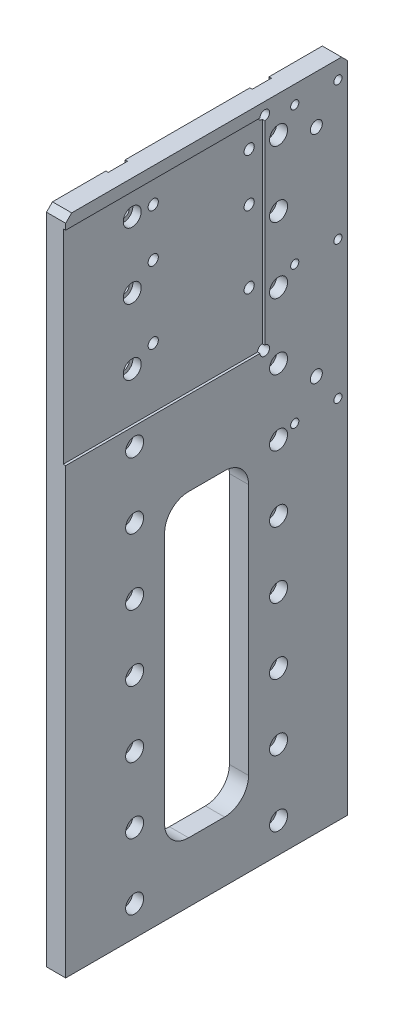
from build123d import *

# Parameters (mm, degrees)
SKETCH_1_W               = 16
SKETCH_1_H               = 550
EXTRUDE_1_DEPTH          = 235
SKETCH_4_W               = 16
SKETCH_4_H               = 550
CUT_EXTRUDE_3_DEPTH      = 2
SKETCH_5_W               = 166
SKETCH_5_H               = 170
CUT_EXTRUDE_4_DEPTH      = 2
HOLE_WIZARD_M10_1_D      = 8.5
HOLE_WIZARD_M10_1_DEPTH  = 27.5
HOLE_WIZARD_M10_1_TIP    = 2.553657631
HOLE_WIZARD_M8_1_D       = 6.8
HOLE_WIZARD_M8_1_DEPTH   = 25
HOLE_WIZARD_M8_1_TIP     = 2.042926105
SKETCH_15_W              = 70
SKETCH_15_H              = 250
CUT_EXTRUDE_5_DEPTH      = 16
FILLET_1_R               = 20
CHAMFER_1_SIZE           = 5
HOLE_WIZARD_1_AT_2_COUNT = 2
HOLE_WIZARD_1_AT_2_PITCH = 120
PATTERN_LINEAR_1_COUNT   = 10
PATTERN_LINEAR_1_PITCH   = 55
HOLE_WIZARD_M8_2_D       = 6.8
HOLE_WIZARD_M8_2_DEPTH   = 22.25
HOLE_WIZARD_M8_2_TIP     = 2.042926105
SKETCH_20_R              = 4
CUT_EXTRUDE_6_DEPTH      = 363.085625232
MM_1_D                   = 10
MM_1_DEPTH               = 10
MM_1_TIP                 = 3.004303095


with BuildPart() as part:
    # 草图1 → 凸台-拉伸1 (new body)
    with BuildSketch(Plane.XY):
        Rectangle(SKETCH_1_W, SKETCH_1_H)
    extrude(amount=EXTRUDE_1_DEPTH)

    # 草图4 → 切除-拉伸3 (cut)
    with BuildSketch(Plane.ZY.offset(8)):
        with Locations((57.5, 0)):
            Rectangle(SKETCH_4_W, SKETCH_4_H)
        with Locations((177.5, 0)):
            Rectangle(SKETCH_4_W, SKETCH_4_H)
    extrude(amount=-CUT_EXTRUDE_3_DEPTH, mode=Mode.SUBTRACT)

    # 草图5 → 切除-拉伸4 (cut)
    with BuildSketch(Plane(origin=(8, 0, 0), x_dir=(0, 0, -1), z_dir=(1, 0, 0))):
        with Locations((-152, 180)):
            Rectangle(SKETCH_5_W, SKETCH_5_H)
    extrude(amount=-CUT_EXTRUDE_4_DEPTH, mode=Mode.SUBTRACT)

    # M10 螺纹孔1
    with Locations(Plane(origin=(6, 0, 0), x_dir=(0, 0, -1), z_dir=(1, 0, 0))):
        with Locations((-160, 245), (-80, 145), (-160, 145), (-80, 245), (-80, 205), (-160, 205)):
            Hole(HOLE_WIZARD_M10_1_D / 2, depth=HOLE_WIZARD_M10_1_DEPTH)
            with Locations((0, 0, -(HOLE_WIZARD_M10_1_DEPTH + HOLE_WIZARD_M10_1_TIP / 2))):  # 118° drill point
                Cone(0, HOLE_WIZARD_M10_1_D / 2, HOLE_WIZARD_M10_1_TIP, mode=Mode.SUBTRACT)

    # M8 螺纹孔1
    with Locations(Plane(origin=(0, -275, 0), x_dir=(-1, 0, 0), z_dir=(0, -1, 0))):
        with Locations((0, -207.5), (0, -72.5), (0, -27.5), (0, -117.5), (0, -162.5)):
            Hole(HOLE_WIZARD_M8_1_D / 2, depth=HOLE_WIZARD_M8_1_DEPTH)
            with Locations((0, 0, -(HOLE_WIZARD_M8_1_DEPTH + HOLE_WIZARD_M8_1_TIP / 2))):  # 118° drill point
                Cone(0, HOLE_WIZARD_M8_1_D / 2, HOLE_WIZARD_M8_1_TIP, mode=Mode.SUBTRACT)

    # 草图15 → 切除-拉伸5 (cut)
    with BuildSketch(Plane.ZY.offset(8)):
        with Locations((117.5, -100)):
            Rectangle(SKETCH_15_W, SKETCH_15_H)
    extrude(amount=-CUT_EXTRUDE_5_DEPTH, mode=Mode.SUBTRACT)

    # 圆角1
    fillet_1_edges = [part.edges().sort_by_distance(p)[0] for p in [
        (0, 25, 152.5),
        (0, -225, 152.5),
        (0, -225, 82.5),
        (0, 25, 82.5),
    ]]
    fillet(fillet_1_edges, radius=FILLET_1_R)

    # 倒角1
    chamfer_1_edges = [part.edges().sort_by_distance(p)[0] for p in [
        (0, 275, 0),
        (0, 275, 235),
    ]]
    chamfer(chamfer_1_edges, length=CHAMFER_1_SIZE)

    # 草图17 → 打孔尺寸(%根据)内六角圆柱头螺钉的类型1 (revolve, cut)
    with BuildSketch(Plane(origin=(8, -250, 57.5), x_dir=(0, 0, -1), z_dir=(0, 1, 0))):
        Polygon((0, 0), (0, 30.203872786), (4.5, 27.5), (4.5, 9), (7.5, 9), (7.5, 0), align=None)
    hole_wizard_1 = revolve(axis=Axis((14.35, -250, 57.5), (-1, 0, 0)), mode=Mode.SUBTRACT)

    # 打孔尺寸(%根据)内六角圆柱头螺钉的类型1 at 2: 打孔尺寸(%根据)内六角圆柱头螺钉的类型1 ×2
    with Locations(*[(0, 0, i * HOLE_WIZARD_1_AT_2_PITCH) for i in range(1, HOLE_WIZARD_1_AT_2_COUNT)]):
        add(hole_wizard_1, mode=Mode.SUBTRACT)

    # 阵列(线性)1: 打孔尺寸(%根据)内六角圆柱头螺钉的类型1 ×10
    with Locations(*[(0, i * PATTERN_LINEAR_1_PITCH, 0) for i in range(1, PATTERN_LINEAR_1_COUNT)]):
        add(hole_wizard_1, mode=Mode.SUBTRACT)

    # 阵列(线性)1 copy 1 sketch → 阵列(线性)1 copy 1 (revolve, cut)
    with BuildSketch(Plane(origin=(8, -195, 177.5), x_dir=(0, 0, -1), z_dir=(0, 1, 0))):
        Polygon((0, 0), (0, 30.203872786), (4.5, 27.5), (4.5, 9), (7.5, 9), (7.5, 0), align=None)
    revolve(axis=Axis((14.35, -195, 177.5), (-1, 0, 0)), mode=Mode.SUBTRACT)

    # 阵列(线性)1 copy 2 sketch → 阵列(线性)1 copy 2 (revolve, cut)
    with BuildSketch(Plane(origin=(8, -140, 177.5), x_dir=(0, 0, -1), z_dir=(0, 1, 0))):
        Polygon((0, 0), (0, 30.203872786), (4.5, 27.5), (4.5, 9), (7.5, 9), (7.5, 0), align=None)
    revolve(axis=Axis((14.35, -140, 177.5), (-1, 0, 0)), mode=Mode.SUBTRACT)

    # 阵列(线性)1 copy 3 sketch → 阵列(线性)1 copy 3 (revolve, cut)
    with BuildSketch(Plane(origin=(8, -85, 177.5), x_dir=(0, 0, -1), z_dir=(0, 1, 0))):
        Polygon((0, 0), (0, 30.203872786), (4.5, 27.5), (4.5, 9), (7.5, 9), (7.5, 0), align=None)
    revolve(axis=Axis((14.35, -85, 177.5), (-1, 0, 0)), mode=Mode.SUBTRACT)

    # 阵列(线性)1 copy 4 sketch → 阵列(线性)1 copy 4 (revolve, cut)
    with BuildSketch(Plane(origin=(8, -30, 177.5), x_dir=(0, 0, -1), z_dir=(0, 1, 0))):
        Polygon((0, 0), (0, 30.203872786), (4.5, 27.5), (4.5, 9), (7.5, 9), (7.5, 0), align=None)
    revolve(axis=Axis((14.35, -30, 177.5), (-1, 0, 0)), mode=Mode.SUBTRACT)

    # 阵列(线性)1 copy 5 sketch → 阵列(线性)1 copy 5 (revolve, cut)
    with BuildSketch(Plane(origin=(8, 25, 177.5), x_dir=(0, 0, -1), z_dir=(0, 1, 0))):
        Polygon((0, 0), (0, 30.203872786), (4.5, 27.5), (4.5, 9), (7.5, 9), (7.5, 0), align=None)
    revolve(axis=Axis((14.35, 25, 177.5), (-1, 0, 0)), mode=Mode.SUBTRACT)

    # 阵列(线性)1 copy 6 sketch → 阵列(线性)1 copy 6 (revolve, cut)
    with BuildSketch(Plane(origin=(8, 80, 177.5), x_dir=(0, 0, -1), z_dir=(0, 1, 0))):
        Polygon((0, 0), (0, 30.203872786), (4.5, 27.5), (4.5, 9), (7.5, 9), (7.5, 0), align=None)
    revolve(axis=Axis((14.35, 80, 177.5), (-1, 0, 0)), mode=Mode.SUBTRACT)

    # 阵列(线性)1 copy 7 sketch → 阵列(线性)1 copy 7 (revolve, cut)
    with BuildSketch(Plane(origin=(8, 135, 177.5), x_dir=(0, 0, -1), z_dir=(0, 1, 0))):
        Polygon((0, 0), (0, 30.203872786), (4.5, 27.5), (4.5, 9), (7.5, 9), (7.5, 0), align=None)
    revolve(axis=Axis((14.35, 135, 177.5), (-1, 0, 0)), mode=Mode.SUBTRACT)

    # 阵列(线性)1 copy 8 sketch → 阵列(线性)1 copy 8 (revolve, cut)
    with BuildSketch(Plane(origin=(8, 190, 177.5), x_dir=(0, 0, -1), z_dir=(0, 1, 0))):
        Polygon((0, 0), (0, 30.203872786), (4.5, 27.5), (4.5, 9), (7.5, 9), (7.5, 0), align=None)
    revolve(axis=Axis((14.35, 190, 177.5), (-1, 0, 0)), mode=Mode.SUBTRACT)

    # 阵列(线性)1 copy 9 sketch → 阵列(线性)1 copy 9 (revolve, cut)
    with BuildSketch(Plane(origin=(8, 245, 177.5), x_dir=(0, 0, -1), z_dir=(0, 1, 0))):
        Polygon((0, 0), (0, 30.203872786), (4.5, 27.5), (4.5, 9), (7.5, 9), (7.5, 0), align=None)
    revolve(axis=Axis((14.35, 245, 177.5), (-1, 0, 0)), mode=Mode.SUBTRACT)

    # M8 螺纹孔2
    with Locations(Plane(origin=(8, 0, 0), x_dir=(0, 0, -1), z_dir=(1, 0, 0))):
        with Locations((-8, 145), (-44, 145), (-8, 260), (-44, 260), (-8, 30), (-44, 30)):
            Hole(HOLE_WIZARD_M8_2_D / 2, depth=HOLE_WIZARD_M8_2_DEPTH)
            with Locations((0, 0, -(HOLE_WIZARD_M8_2_DEPTH + HOLE_WIZARD_M8_2_TIP / 2))):  # 118° drill point
                Cone(0, HOLE_WIZARD_M8_2_D / 2, HOLE_WIZARD_M8_2_TIP, mode=Mode.SUBTRACT)

    # 草图20 → 切除-拉伸6 (cut, through all)
    with BuildSketch(Plane(origin=(8, 0, 0), x_dir=(0, 0, -1), z_dir=(1, 0, 0))):
        with Locations(Location((-69, 95, 0), (0, 0, 331.044975628))):
            Circle(SKETCH_20_R)
        with Locations(Location((-69, 265, 0), (0, 0, 28.955024372))):
            Circle(SKETCH_20_R)
    extrude(amount=-CUT_EXTRUDE_6_DEPTH, mode=Mode.SUBTRACT)

    # 大小mm 暗销孔1
    with Locations(Plane(origin=(8, 0, 0), x_dir=(0, 0, -1), z_dir=(1, 0, 0))):
        with Locations((-26, 235), (-26, 55)):
            Hole(MM_1_D / 2, depth=MM_1_DEPTH)
            with Locations((0, 0, -(MM_1_DEPTH + MM_1_TIP / 2))):  # 118° drill point
                Cone(0, MM_1_D / 2, MM_1_TIP, mode=Mode.SUBTRACT)


solid = part.part
